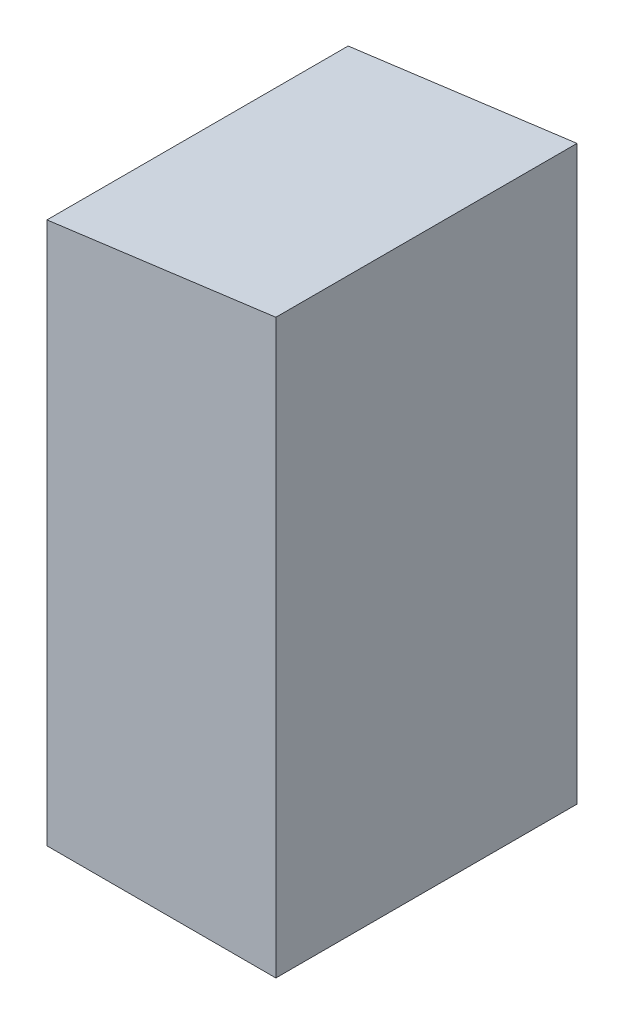
SolidWorks part; units mm, degrees
ref_plane "Front Plane" through (0, 0, 0) normal (0, 0, 1) x (1, 0, 0)
ref_plane "Top Plane" through (0, 0, 0) normal (0, 1, 0) x (1, 0, 0)
ref_plane "Right Plane" through (0, 0, 0) normal (1, 0, 0) x (0, 0, -1)
sketch "Sketch1" plane through (0, 0, 0) normal (0, 0, 1) x (1, 0, 0)
  line L0 (0, 45) -> (19, 47.5)
  line L1 (0, 0) -> (19, 0)
  line L2 (0, 0) -> (0, 45)
  line L4 (19, 0) -> (19, 47.5)
  dimension "D1" = 47.5
  dimension "D2" = 45
  dimension "D3" = 19
extrude "Boss-Extrude1" add sketch "Sketch1" along normal blind 25
